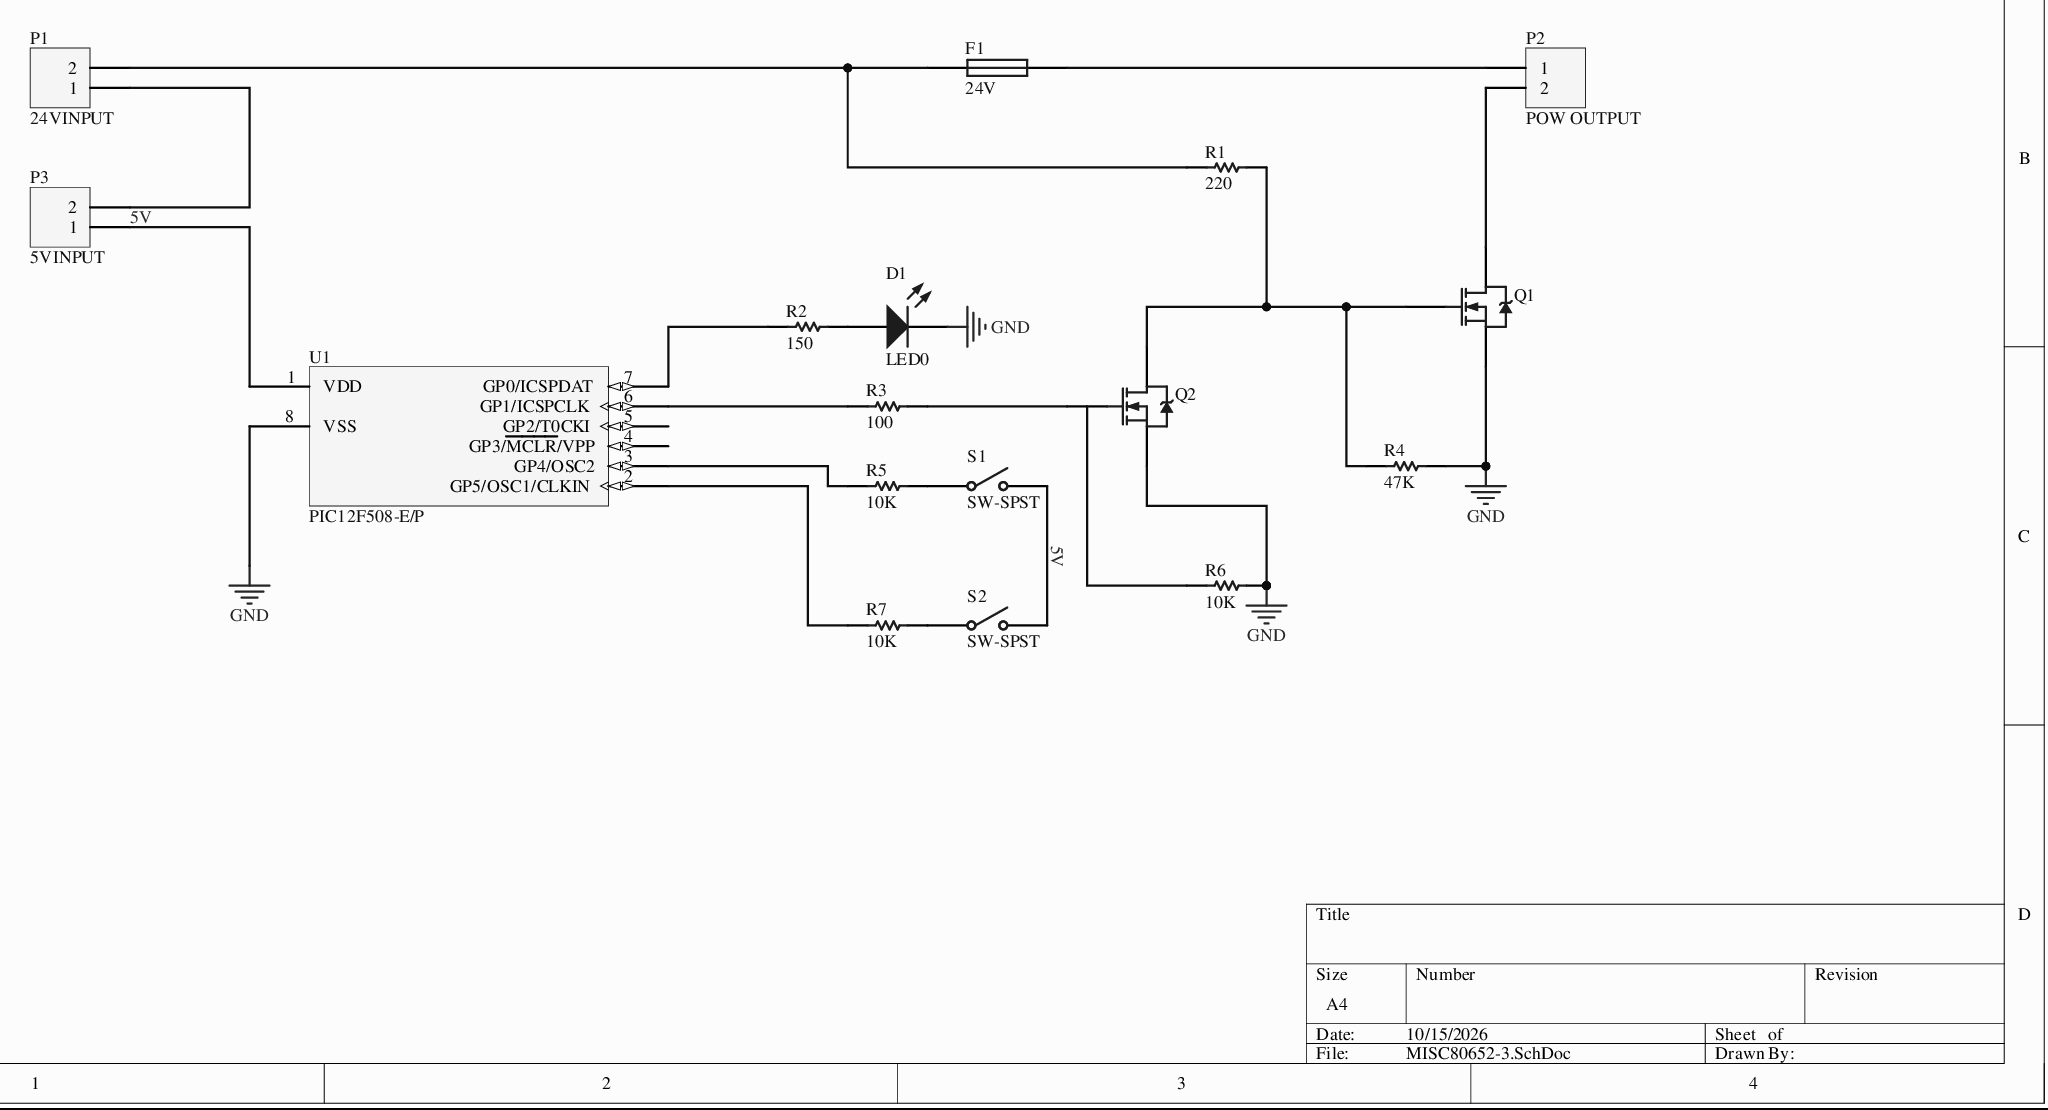
[diagram p0: MISC80652-3.SchDoc]
# Altium project MISC80652-6.PrjPcb
1 sheet, 17 parts. Net scope: global (net labels, ports and power ports of the same name join across sheets).
Board file: MISC80652.PcbDoc

## Sheet MISC80652-3.SchDoc
size A4

### Parts
D1  LED0  [LED-0]
F1  24V  [PIN-W2/E2.8]
P1  24VINPUT  [HDR1X2]
P2  POW OUTPUT  [HDR1X2]
P3  5VINPUT  [HDR1X2]
Q1  JANTXV2N7224  [TO-254AA]  (value not drawn)
Q2  JANTXV2N7224  [TO-254AA]  (value not drawn)
R1  220  [AXIAL-0.3]
R2  150  [AXIAL-0.3]
R3  100  [AXIAL-0.3]
R4  47K  [AXIAL-0.3]
R5  10K  [AXIAL-0.3]
R6  10K  [AXIAL-0.3]
R7  10K  [AXIAL-0.3]
S1  SW-SPST  [SPST-2]
S2  SW-SPST  [SPST-2]
U1  PIC12F508-E/P  [PDIP300-P8]

### Nets
GND: D1.2(K) Q1.2(S) Q2.2(S) R4.2 R6.2 U1.8(VSS)
5V: P3.1 S1.2(NO) S2.2(NO) U1.1(VDD)
NetD1_1: D1.1(A) R2.2
NetF1_1: F1.1 P1.2 R1.1
NetF1_2: F1.2 P2.1
NetP1_1: P1.1 P3.2
NetP2_2: P2.2 Q1.1(D)
NetQ1_3: Q1.3(G) Q2.1(D) R1.2 R4.1
NetQ2_3: Q2.3(G) R3.2
NetR2_1: R2.1 U1.7(GP0/ICSPDAT)
NetR3_1: R3.1 U1.6(GP1/ICSPCLK)
NetR5_1: R5.1 U1.3(GP4/OSC2)
NetR5_2: R5.2 S1.1(COMMON)
NetR7_1: R7.1 U1.2(GP5/OSC1/CLKIN)
NetR7_2: R7.2 S2.1(COMMON)

Not connected (* = marked no-connect by the designer): R6 1; U1 4(GP3/~{MCLR}/VPP) 5(GP2/T0CKI)

### Library data of the parts
D1 = LED0: Typical INFRARED GaAs LED; Published: 8-Jun-2000; LatestRevisionDate: 08-Jul-2005; LatestRevisionNote: Mech Layer 1 removed.; PackageReference: LED-0; PackageDescription: LED; 2 Leads; Publisher: Altium Limited
F1 = Fuse 1: Fuse; Published: 8-Jun-2000; LatestRevisionDate: 17-Jul-2002; LatestRevisionNote: Re-released for DXP Platform.; PackageReference: PIN-W2/E2.8; PackageDescription: Thru-Hole; 2 Leads; Publisher: Altium Limited
P1-P3 = Header 2: Header, 2-Pin; LatestRevisionDate: 17-Jul-2002; LatestRevisionNote: Re-released for DXP Platform.; Publisher: Altium Limited
Q1 Q2 = JANTXV2N7224: HEXFET Power MOSFET; Code - JEDEC: TO-254-AA; Published: 17-Sep-2003; Datasheet: Latest Revision: PD-9.487C; Package Reference: TO-254AA; Publisher: Altium Limited
R1-R7 = Res1: Resistor; Value: 1K; Published: 8-Jun-2000; LatestRevisionDate: 17-Jul-2002; LatestRevisionNote: Re-released for DXP Platform.; PackageReference: AXIAL-0.3; PackageDescription: Axial Device, Thru-Hole; 2 Leads; 0.3 in Pin Spacing; Publisher: Altium Limited
S1 S2 = SW-SPST: Single-Pole, Single-Throw Switch; Published: 24-Mar-1999; LatestRevisionDate: 17-Jul-2002; LatestRevisionNote: Re-released for DXP Platform.; PackageReference: SPST-2; PackageDescription: Switch; 2 Leads; Publisher: Altium Limited
U1 = PIC12F508-E/P: 8-bit Flash Microcontroller, 512 (x12-Bit words) Program Memory, 25 Bytes Data Memory, 8-Pin PDIP, Extended Temperature; Published: 29-Jan-2009; LatestRevisionDate: 02-Dec-2009; LatestRevisionNote: Updated to datasheet revision revE, Aug-2009; DatasheetVersion: revE, Aug-2009; PackageVersion: revBB, Aug-2009; PackageReference: PDIP300-P8; PackageDescription: 8-Lead Plastic Dual In-Line (P) - 300 mil Body [PDIP]; Supplier 1: Digi-Key; Supplier Part Number 1: PIC12F508-E/P-ND; Supplier 2: Farnell; Supplier Part Number 2: 1816016; Code_JEDEC: MS-001; ComponentLink1Description: Datasheet; ComponentLink1URL: http://ww1.microchip.com/downloads/en/DeviceDoc/41236E.pdf; ComponentLink2Description: Packaging Specification; ComponentLink2URL: http://www.microchip.com/stellent/groups/techpub_sg/documents/packagingspec/en012702.pdf; ComponentLink3Description: Microchip.com Home; ComponentLink3URL: http://www.microchip.com/; Publisher: Altium Limited